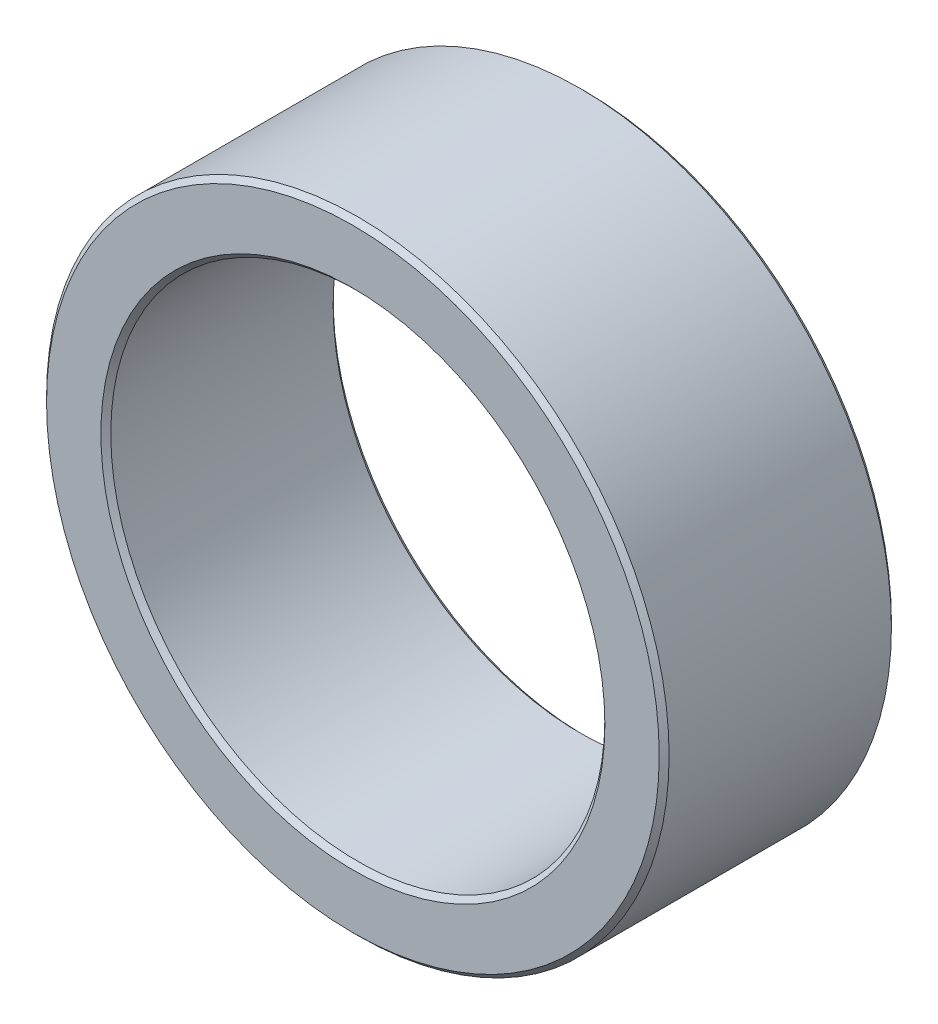
SolidWorks part; units mm, degrees
material "普通碳钢"
ref_plane "前视基准面" through (0, 0, 0) normal (0, 0, 1) x (1, 0, 0)
ref_plane "上视基准面" through (0, 0, 0) normal (0, 1, 0) x (1, 0, 0)
ref_plane "右视基准面" through (0, 0, 0) normal (1, 0, 0) x (0, 0, -1)
sketch "草图1" plane through (0, 0, 0) normal (0, 0, 1) x (1, 0, 0)
  circle A0 centre (0, 0) radius 25
  circle A1 centre (0, 0) radius 31.5
  dimension "D1" = 50
  dimension "D2" = 63
extrude "凸台-拉伸1" add sketch "草图1" along normal blind 23.5
chamfer "倒角1" distance 0.5 angle 45 4 edges at (25, 0, 0) (31.5, 0, 0) (25, 0, 23.5) (31.5, 0, 23.5)
